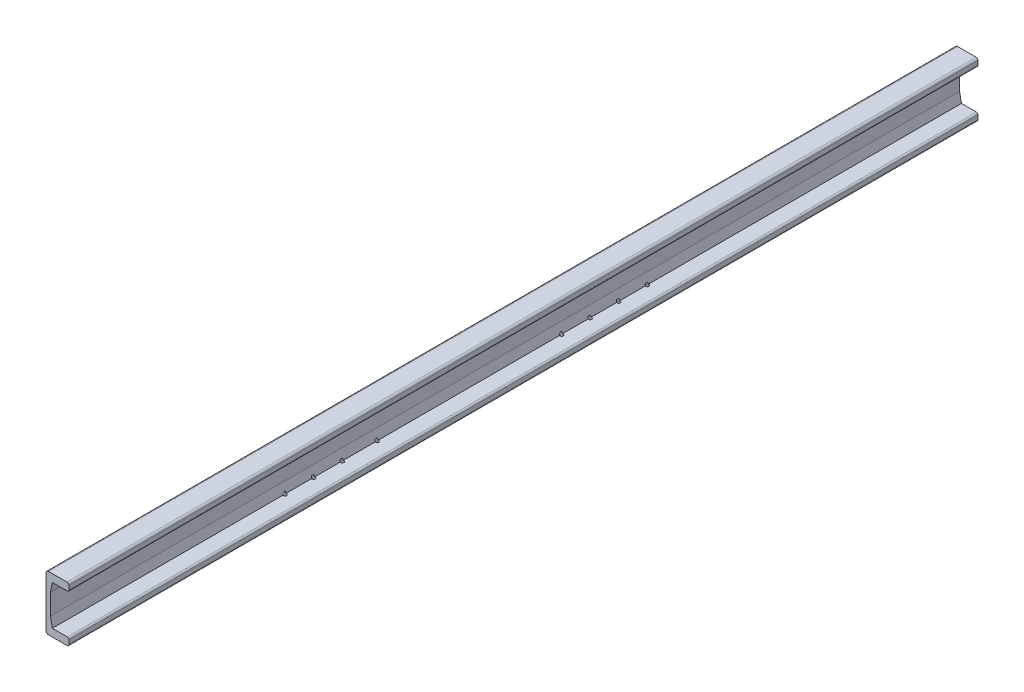
SolidWorks part; units mm, degrees
material "1023 碳钢板 (SS)"
ref_plane "Front Plane" through (0, 0, 0) normal (0, 0, 1) x (1, 0, 0)
ref_plane "Top Plane" through (0, 0, 0) normal (0, 1, 0) x (1, 0, 0)
ref_plane "Right Plane" through (0, 0, 0) normal (1, 0, 0) x (0, 0, -1)
sketch "Sketch1" plane through (0, 0, 0) normal (0, 0, 1) x (1, 0, 0)
  line L0 (-3, 0) -> (-32, 0)
  line L1 (-36, -4) -> (-36, -82.5)
  line L2 (-32, -86.5) -> (-3, -86.5)
  line L3 (0, -83.5) -> (0, -77)
  line L4 (-2.5, -74.5) -> (-26, -74.5)
  line L5 (-29, -59.5) -> (-29, -27)
  line L6 (-26, -12) -> (-2.5, -12)
  line L7 (0, -9.5) -> (0, -3)
  line L8 (-29, -27) -> (-26, -12)
  line L9 (-26, -74.5) -> (-29, -59.5)
  arc A0 (-3, -86.5) -> (0, -83.5) centre (-3, -83.5) ccw
  arc A1 (-3, 0) -> (0, -3) centre (-3, -3) cw
  arc A2 (0, -77) -> (-2.5, -74.5) centre (-2.5, -77) ccw
  arc A3 (-2.5, -12) -> (0, -9.5) centre (-2.5, -9.5) ccw
  arc A4 (-36, -82.5) -> (-32, -86.5) centre (-32, -82.5) ccw
  arc A5 (-32, 0) -> (-36, -4) centre (-32, -4) ccw
  point P15 (0, -86.5)
  point P18 (0, 0)
  point P21 (0, -74.5)
  point P24 (0, -12)
  point P27 (-36, -86.5)
  point P30 (-36, 0)
  dimension "D10" = 3
  dimension "D11" = 2.5
  dimension "D12" = 4
  dimension "D1" = 86.5
  dimension "D2" = 12
  dimension "D3" = 12
  dimension "D4" = 36
  dimension "D5" = 7
  dimension "D6" = 15
  dimension "D7" = 15
  dimension "D8" = 3
  dimension "D9" = 3
extrude "Boss-Extrude1" add sketch "Sketch1" along normal blind 1430 contours L7 A1 L0 A5 L1 A4 L2 A0 L3 A2 L4 L9 L5 L8 L6 A3
sketch "Sketch2" plane through (0, -86.5, 0) normal (0, -1, 0) x (1, 0, 0)
  line L0 (0, 1430) -> (0, 0) construction
  line L1 (-32, 1430) -> (-3, 1430) construction
  circle A1 centre (-25, 495) radius 2
  circle A2 centre (-25, 540) radius 2
  circle A3 centre (-25, 975) radius 2
  circle A4 centre (-25, 585) radius 2
  circle A5 centre (-25, 630) radius 2
  circle A6 centre (-25, 1065) radius 2
  circle A7 centre (-25, 920) radius 2
  circle A8 centre (-25, 1020) radius 2
  dimension "D3" = 135
  dimension "D10" = 4
  dimension "D1" = 45
  dimension "D2" = 90
  dimension "D4" = 145
  dimension "D5" = 45
  dimension "D6" = 45
  dimension "D7" = 290
  dimension "D8" = 25
  dimension "D9" = 365
extrude "Cut-Extrude1" cut sketch "Sketch2" against normal blind 10
hole_wizard "M6 Tapped Hole1" positions "Sketch3" profile "Sketch4" tap size "M6" standard "ISO"
sketch "Sketch3" plane through (0, -86.5, 0) normal (0, -1, 0) x (-1, 0, 0)
  point P0 (25, -630)
  point P3 (25, -585)
  point P6 (25, -540)
  point P9 (25, -495)
  point P12 (25, -920)
  point P15 (25, -975)
  point P18 (25, -1020)
  point P21 (25, -1065)
sketch "Sketch4" plane through (-25, -86.5, 630) normal (1, 0, 0) x (0, 0, -1)
  line L0 (0, 0) -> (0, 16.5022)
  line L1 (0, 16.5022) -> (2.5, 15)
  line L2 (2.5, 15) -> (2.5, 0)
  line L5 (2.5, 0) -> (0, 0)
  line L10 (0, 16.5022) -> (-2.5, 15) construction
  line L11 (0, -6.35) -> (0, 107.95) construction
  dimension "螺纹孔钻头直径" = 5
  dimension "螺纹孔钻头深度" = 15
  dimension "导头角度" = 118
cosmetic thread "Hole thread line 1" parameters "D1"=12, "D2"=6
cosmetic thread "Hole thread line 2" parameters "D1"=12, "D2"=6
cosmetic thread "Hole thread line 3" parameters "D1"=12, "D2"=6
cosmetic thread "Hole thread line 4" parameters "D1"=12, "D2"=6
cosmetic thread "Hole thread line 5" parameters "D1"=12, "D2"=6
cosmetic thread "Hole thread line 6" parameters "D1"=12, "D2"=6
cosmetic thread "Hole thread line 7" parameters "D1"=12, "D2"=6
cosmetic thread "Hole thread line 8" parameters "D1"=12, "D2"=6
